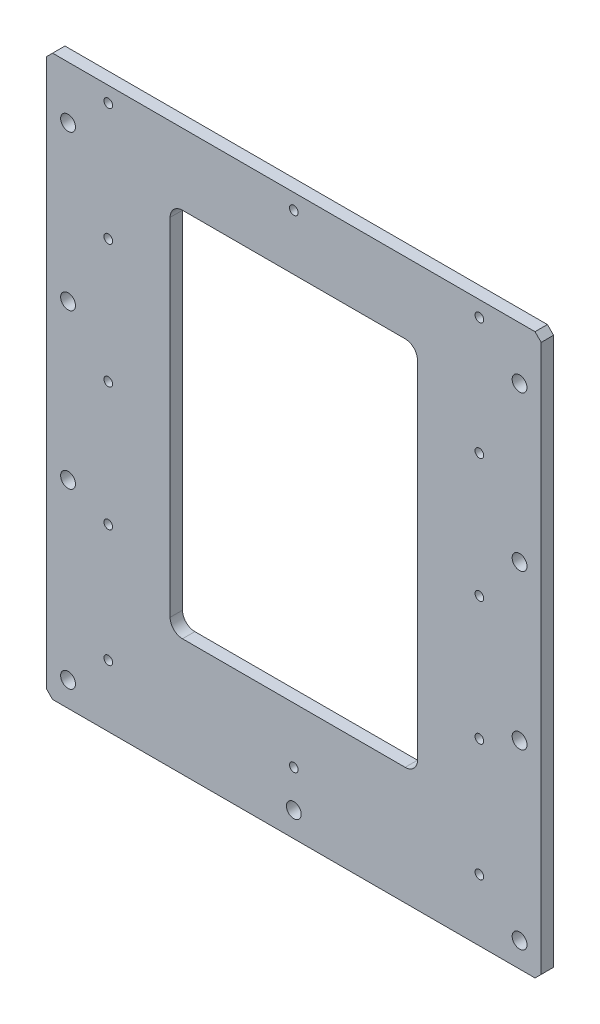
SolidWorks part; units mm, degrees
material "Q235A"
ref_plane "前视基准面" through (0, 0, 0) normal (0, 0, 1) x (1, 0, 0)
ref_plane "上视基准面" through (0, 0, 0) normal (0, 1, 0) x (1, 0, 0)
ref_plane "右视基准面" through (0, 0, 0) normal (1, 0, 0) x (0, 0, -1)
sketch "草图1" plane through (0, 0, 0) normal (0, 0, 1) x (1, 0, 0)
  line L1 (-400, 490) -> (400, 490)
  line L2 (-400, 490) -> (-400, -490)
  line L3 (-400, -490) -> (400, -490)
  line L4 (400, 490) -> (400, -490)
  line L5 (0, -490) -> (0, 490) construction
  line L6 (-400, 0) -> (400, 0) construction
  point P0 (0, 0)
  dimension "D1" = 800
  dimension "D2" = 980
extrude "凸台-拉伸1" add sketch "草图1" along normal blind 20
hole_wizard "M16 螺纹孔1" positions "草图2" profile "草图3" tap size "M16" standard "GB"
sketch "草图2" plane through (0, 0, 20) normal (0, 0, 1) x (1, 0, 0)
  line L1 (-300, -390) -> (300, -390) construction
  line L2 (-300, -390) -> (-300, 390) construction
  line L3 (-300, 390) -> (300, 390) construction
  line L4 (300, -390) -> (300, 390) construction
  line L5 (0, 390) -> (0, -390) construction
  line L6 (-300, 0) -> (300, 0) construction
  line L7 (-300, 200) -> (300, 200) construction
  line L8 (-300, -200) -> (300, -200) construction
  point P2 (300, 390)
  point P351 (-300, -390)
  point P352 (-300, 390)
  point P353 (300, -390)
  point P354 (-300, 0)
  point P355 (0, -390)
  point P356 (300, 0)
  point P357 (0, 390)
  point P360 (-300, 200)
  point P361 (300, 200)
  point P362 (-300, -200)
  point P363 (300, -200)
  dimension "D1" = 600
  dimension "D2" = 780
  dimension "D3" = 400
sketch "草图3" plane through (300, 390, 20) normal (1, 0, 0) x (0, -1, 0)
  line L0 (0, 0) -> (0, 46.206)
  line L1 (0, 46.206) -> (7, 42)
  line L2 (7, 42) -> (7, 0)
  line L5 (7, 0) -> (0, 0)
  line L10 (0, 46.206) -> (-7, 42) construction
  line L11 (0, -6.35) -> (0, 107.95) construction
  dimension "螺纹孔钻头直径" = 14
  dimension "螺纹孔钻头深度" = 42
  dimension "导头角度" = 118
cosmetic thread "孔螺蚊线1" parameters "D1"=20, "D2"=16
cosmetic thread "孔螺蚊线2" parameters "D1"=20, "D2"=16
cosmetic thread "孔螺蚊线3" parameters "D1"=20, "D2"=16
cosmetic thread "孔螺蚊线4" parameters "D1"=20, "D2"=16
cosmetic thread "孔螺蚊线5" parameters "D1"=20, "D2"=16
cosmetic thread "孔螺蚊线6" parameters "D1"=20, "D2"=16
cosmetic thread "孔螺蚊线7" parameters "D1"=20, "D2"=16
cosmetic thread "孔螺蚊线8" parameters "D1"=20, "D2"=16
cosmetic thread "孔螺蚊线9" parameters "D1"=20, "D2"=16
cosmetic thread "孔螺蚊线10" parameters "D1"=20, "D2"=16
cosmetic thread "孔螺蚊线11" parameters "D1"=20, "D2"=16
cosmetic thread "孔螺蚊线12" parameters "D1"=20, "D2"=16
sketch "草图4" plane through (0, 0, 20) normal (0, 0, 1) x (1, 0, 0)
  line L1 (-200, -300) -> (200, -300)
  line L2 (-200, -300) -> (-200, 300)
  line L3 (-200, 300) -> (200, 300)
  line L4 (200, -300) -> (200, 300)
  line L5 (0, 300) -> (0, -300) construction
  line L6 (-200, 0) -> (200, 0) construction
  point P0 (0, 0)
  dimension "D1" = 400
  dimension "D2" = 600
extrude "切除-拉伸1" cut sketch "草图4" against normal blind 20
fillet "圆角1" radius 20 4 edges at (-200, -300, 10) (200, -300, 10) (200, 300, 10) (-200, 300, 10)
sketch "草图10" plane through (0, 0, 20) normal (0, 0, 1) x (1, 0, 0)
  line L0 (400, -490) -> (400, 490) construction
  line L1 (-400, 490) -> (400, 490)
  line L2 (-400, 490) -> (-400, 415)
  line L3 (-400, 415) -> (400, 415)
  line L4 (400, 490) -> (400, 415)
  circle A0 centre (0, 390) radius 7 construction
  dimension "D1" = 25
extrude "切除-拉伸3" cut sketch "草图10" against normal through all
hole_wizard "Ø24.0 (24) 直径孔1" positions "草图7" profile "草图8" hole size "Ø24.0" standard "GB" end condition through all
sketch "草图7" plane through (0, 0, 20) normal (0, 0, 1) x (1, 0, 0)
  line L1 (365, -450) -> (-365, -450) construction
  line L2 (365, -450) -> (365, 450) construction
  line L3 (365, 450) -> (-365, 450) construction
  line L4 (-365, -450) -> (-365, 450) construction
  line L5 (0, 450) -> (0, -450) construction
  line L6 (365, 0) -> (-365, 0) construction
  line L7 (-365, 330) -> (365, 330) construction
  line L8 (-365, 80) -> (365, 80) construction
  line L9 (-365, -170) -> (365, -170) construction
  circle A1 centre (-300, 390) radius 7 construction
  point P111 (365, -450)
  point P113 (-365, -450)
  point P115 (0, -450)
  point P117 (0, 450)
  point P141 (-365, 330)
  point P142 (365, 330)
  point P143 (-365, 80)
  point P162 (-365, -170)
  point P164 (365, -170)
  point P189 (365, 80)
  dimension "D4" = 250
  dimension "D1" = 730
  dimension "D2" = 900
  dimension "D3" = 250
  dimension "D5" = 60
sketch "草图8" plane through (365, 80, 20) normal (1, 0, 0) x (0, -1, 0)
  line L0 (0, 0) -> (0, 20)
  line L1 (0, 20) -> (12, 20)
  line L2 (12, 20) -> (12, 0)
  line L5 (12, 0) -> (0, 0)
  line L11 (0, -6.35) -> (0, 107.95) construction
  dimension "通孔孔直径" = 24
  dimension "通孔孔深度" = 20
chamfer "倒角1" distance 10 angle 45 4 edges at (400, -490, 10) (-400, -490, 10) (-400, 415, 10) (400, 415, 10)
